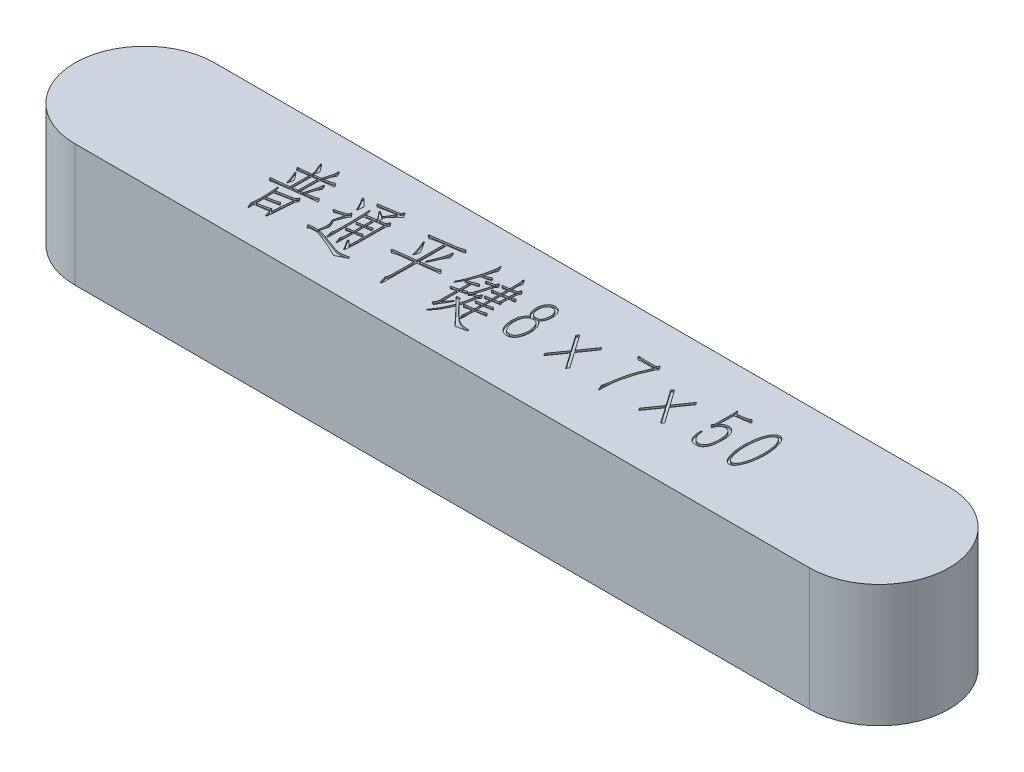
SolidWorks part; units mm, degrees
ref_plane "Front Plane" through (0, 0, 0) normal (0, 0, 1) x (1, 0, 0)
ref_plane "Top Plane" through (0, 0, 0) normal (0, 1, 0) x (1, 0, 0)
ref_plane "Right Plane" through (0, 0, 0) normal (1, 0, 0) x (0, 0, -1)
sketch "Sketch1" plane through (0, 0, 0) normal (0, 1, 0) x (1, 0, 0)
  line L0 (0, 0) -> (42, 0) construction
  line L1 (0, 4) -> (42, 4)
  line L2 (0, -4) -> (42, -4)
  arc A0 (0, 4) -> (0, -4) centre (0, 0) ccw
  arc A1 (42, -4) -> (42, 4) centre (42, 0) ccw
  point P3 (21, 0)
  point P8 (-4, 0)
  point P9 (46, 0)
extrude "Boss-Extrude1" add sketch "Sketch1" along normal blind 7
sketch "Sketch2" plane through (0, 7, 0) normal (0, 1, 0) x (1, 0, 0)
  line L0 (0, -1.4184) -> (42.3836, -1.4184) construction
  text T0 "普通平键8×7×50" font "汉仪长仿宋体" height in points 12
extrude "Cut-Extrude1" cut sketch "Sketch2" against normal blind 0.1
equation "\"b\"= 8"
equation "\"h\"= 7"
equation "\"l\"= 50"
equation "\"D1@Sketch1\"=\"b\"/2"
equation "\"D2@Sketch1\"=\"l\""
equation "\"D1@Boss-Extrude1\"=\"h\""
